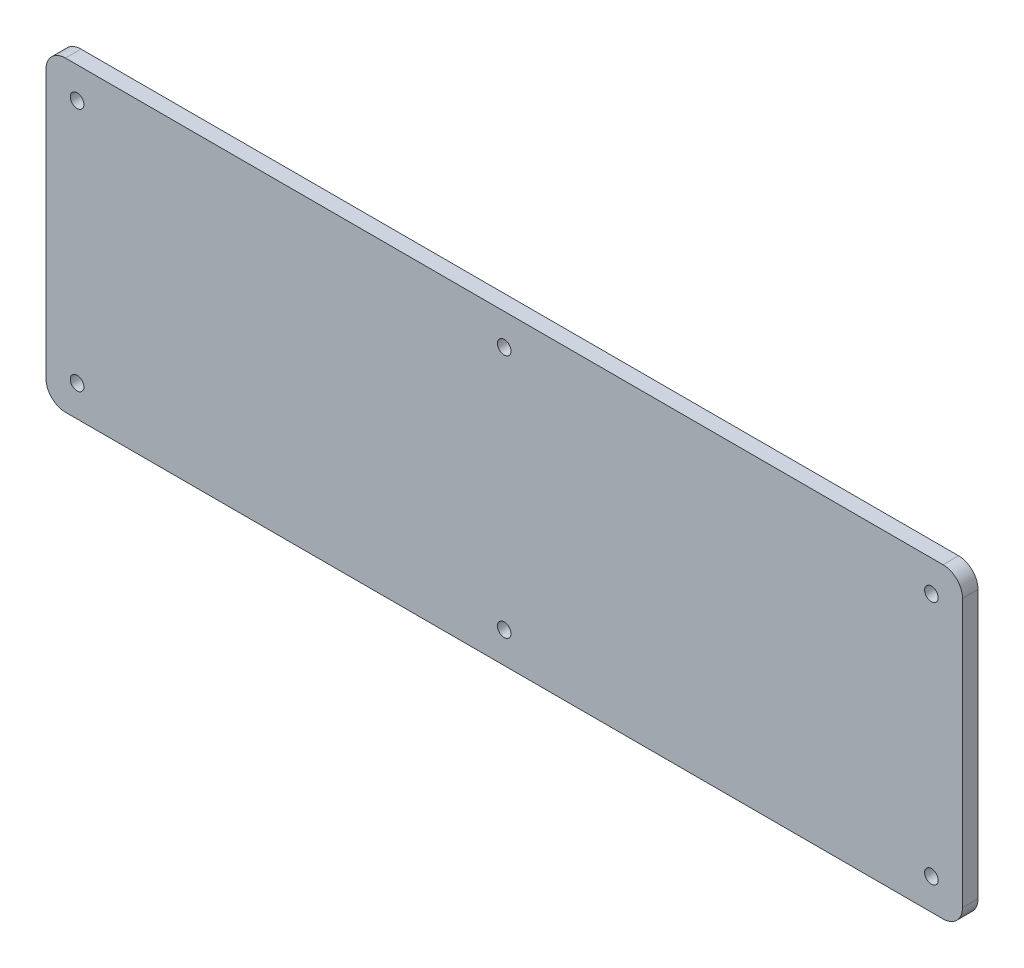
SolidWorks part; units mm, degrees
ref_plane "Front Plane" through (0, 0, 0) normal (0, 0, 1) x (1, 0, 0)
ref_plane "Top Plane" through (0, 0, 0) normal (0, 1, 0) x (1, 0, 0)
ref_plane "Right Plane" through (0, 0, 0) normal (1, 0, 0) x (0, 0, -1)
sketch "Sketch1" plane through (0, 0, 0) normal (0, 0, 1) x (1, 0, 0)
  line L1 (118, -39.5) -> (-118, -39.5)
  line L2 (118, -39.5) -> (118, 39.5)
  line L3 (118, 39.5) -> (-118, 39.5)
  line L4 (-118, -39.5) -> (-118, 39.5)
  line L5 (118, -39.5) -> (-118, 39.5) construction
  line L6 (118, 39.5) -> (-118, -39.5) construction
  point P0 (0, 0)
  dimension "D1" = 236
  dimension "D2" = 79
extrude "Boss-Extrude1" add sketch "Sketch1" along normal blind 4
fillet "Fillet1" radius 5 4 edges at (118, 39.5, 2) (118, -39.5, 2) (-118, -39.5, 2) (-118, 39.5, 2)
sketch "Sketch4" plane through (0, 0, 0) normal (0, 0, -1) x (-1, 0, 0)
  line L1 (-110, -31.5) -> (110, -31.5) construction
  line L2 (-110, -31.5) -> (-110, 31.5) construction
  line L3 (-110, 31.5) -> (110, 31.5) construction
  line L4 (110, -31.5) -> (110, 31.5) construction
  line L5 (-110, -31.5) -> (110, 31.5) construction
  line L6 (-110, 31.5) -> (110, -31.5) construction
  line L7 (-113, 39.5) -> (113, 39.5) construction
  line L8 (118, 34.5) -> (118, -34.5) construction
  circle A0 centre (-110, 31.5) radius 1.75
  circle A1 centre (110, 31.5) radius 1.75
  circle A2 centre (110, -31.5) radius 1.75
  circle A3 centre (-110, -31.5) radius 1.75
  circle A4 centre (0, 31.5) radius 1.75
  circle A5 centre (0, -31.5) radius 1.75
  point P0 (0, 0)
  dimension "D3" = 3.5
  dimension "D1" = 8
  dimension "D2" = 8
extrude "Cut-Extrude1" cut sketch "Sketch4" against normal through all
